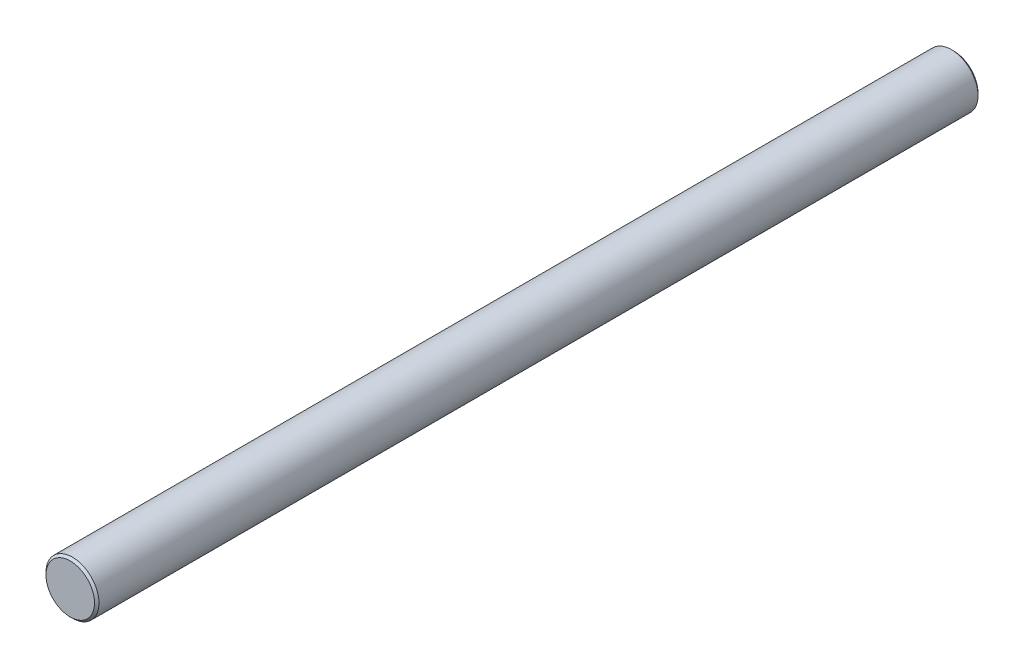
from build123d import *

# Parameters (mm, degrees)
SKETCH_1_R      = 6
EXTRUDE_1_DEPTH = 100
CHAMFER_1_SIZE  = 0.5


with BuildPart() as part:
    # 草图1 → 凸台-拉伸1 (new, symmetric)
    with BuildSketch(Plane.XY):
        Circle(SKETCH_1_R)
    extrude(amount=EXTRUDE_1_DEPTH, both=True)

    # 倒角1
    chamfer_1_edges = [part.edges().sort_by_distance(p)[0] for p in [
        (-6, 0, -100),
        (-6, 0, 100),
    ]]
    chamfer(chamfer_1_edges, length=CHAMFER_1_SIZE)


solid = part.part
